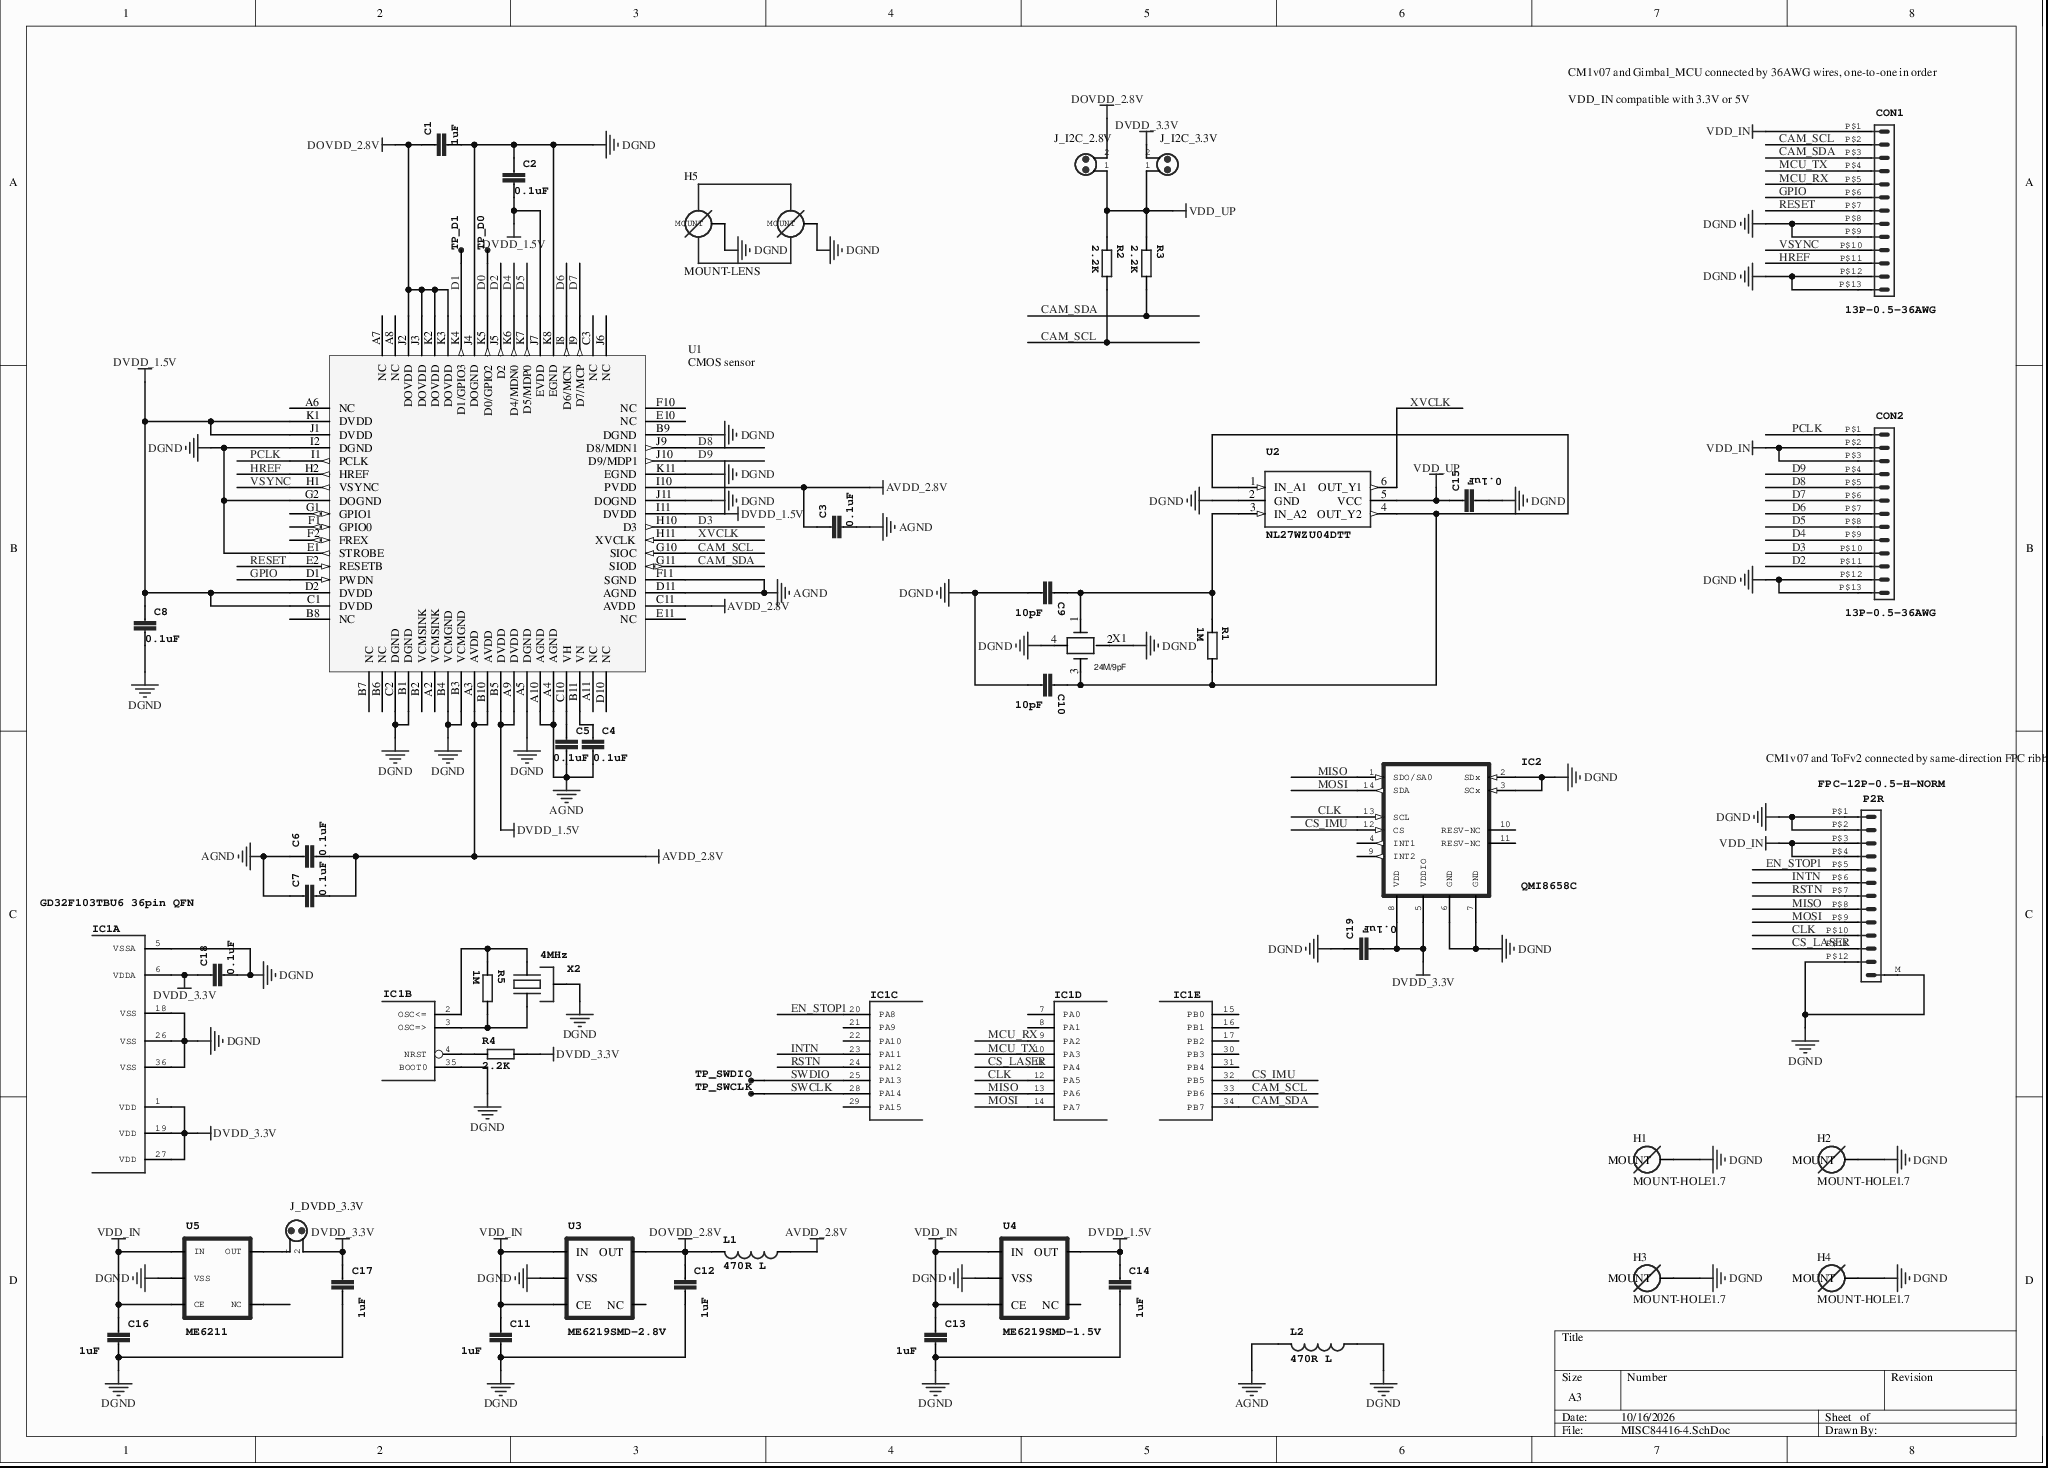
[diagram p0: MISC84416-4.SchDoc]
# Altium project MISC84416-3.PrjPcb
1 sheet, 50 parts. Net scope: global (net labels, ports and power ports of the same name join across sheets).
Board file: MISC84416.PcbDoc

## Sheet MISC84416-4.SchDoc
size A3

### Parts
C1  1uF  [RCL_C0402_TI]
C2  0.1uF  [RCL_C0402_TI]
C3  0.1uF  [RCL_C0402_TI]
C4  0.1uF  [RCL_C0402_TI]
C5  0.1uF  [RCL_C0402_TI]
C6  0.1uF  [RCL_C0402_TI]
C7  0.1uF  [RCL_C0402_TI]
C8  0.1uF  [RCL_C0402_TI]
C9  10pF  [RCL_C0402_TI]
C10  10pF  [RCL_C0402_TI]
C11  1uF  [RCL_C0402_TI]
C12  1uF  [RCL_C0402_TI]
C13  1uF  [RCL_C0402_TI]
C14  1uF  [RCL_C0402_TI]
C15  0.1uF  [RCL_C0402_TI]
C16  1uF  [RCL_C0402_TI]
C17  1uF  [RCL_C0402_TI]
C18  0.1uF  [RCL_C0402_TI]
C19  0.1uF  [RCL_C0402_TI]
CON1  13P-0.5-36AWG  [13P-0.5-36AWG]
CON2  13P-0.5-36AWG  [13P-0.5-36AWG]
H1  MOUNT-HOLE1.7  [MOUNT-HOLE1.7]
H2  MOUNT-HOLE1.7  [MOUNT-HOLE1.7]
H3  MOUNT-HOLE1.7  [MOUNT-HOLE1.7]
H4  MOUNT-HOLE1.7  [MOUNT-HOLE1.7]
H5  MOUNT-LENS  [MOUNT-LENS-M12-1.6]
IC1  GD32F103TBU6 36pin QFN  [GD32_QFN36]  (parts A,B,C,D,E of 5)
IC2  QMI8658C  [LGA14_3X2.5]
J_DVDD_3.3V  JUMPER_2P_MIN  [JUMPER_2P_MIN]  (value not drawn)
J_I2C_2.8V  JUMPER_2P_MIN  [JUMPER_2P_MIN]  (value not drawn)
J_I2C_3.3V  JUMPER_2P_MIN  [JUMPER_2P_MIN]  (value not drawn)
L1  470R L  [RCL_L0603]
L2  470R L  [RCL_L0603]
P2R  FPC-12P-0.5-H-NORM  [FPC-12P-0.5-H-NORM]
R1  1M  [RCL_R0402_TI]
R2  2.2K  [RCL_R0402_TI]
R3  2.2K  [RCL_R0402_TI]
R4  2.2K  [RCL_R0402_TI]
R5  1M  [RCL_R0402_TI]
TP_D0  (no value)  [TP-1]
TP_D1  (no value)  [TP-1]
TP_SWCLK  (no value)  [TP-1]
TP_SWDIO  (no value)  [TP-1]
U1  CMOS sensor  [BGA71_5.99X5.84]
U2  NL27WZU04DTT  [SOT23-6]
U3  ME6219SMD-2.8V  [SOT23-5]
U4  ME6219SMD-1.5V  [SOT23-5]
U5  ME6211  [SOT23-5]
X1  24M/9pF  [EPSON-TSX3225]
X2  4MHz  [XTAL_4.5X2.0]

### Nets
AGND: C3.2 C4.2 C5.2 C6.1 C7.1 L2.2 U1.A4(AGND) U1.A10(AGND) U1.D11(AGND) U1.F11(SGND)
AVDD_2.8V: C3.1 C6.2 C7.2 L1.1 U1.A3(AVDD) U1.B10(AVDD) U1.C11(AVDD) U1.I10(PVDD)
DGND: C1.2 C2.1 C8.2 C9.2 C10.2 C11.2 C12.2 C13.2 C14.2 C15.2 C16.2 C17.2 C18.2 C19.1 CON1.P$8 CON1.P$9 CON1.P$12 CON1.P$13 CON2.P$12 CON2.P$13 H1.MOUNT H2.MOUNT H3.MOUNT H4.MOUNT H5.MOUNT IC1.5(VSSA) IC1.18(VSS) IC1.26(VSS) IC1.35(BOOT0) IC1.36(VSS) IC2.2(SDx) IC2.3(SCx) IC2.6(GND) IC2.7(GND) L2.1 P2R.M P2R.P$1 P2R.P$2 P2R.P$12 U1.A5(DGND) U1.B1(DGND) U1.B3(VCMGND) U1.B4(VCMGND) U1.B9(DGND) U1.C2(DGND) U1.E1(STROBE) U1.G2(DOGND) U1.I2(DGND) U1.J4(DOGND) U1.J11(DOGND) U1.K8(EGND) U1.K11(EGND) U2.2(GND) U3.2(VSS) U4.2(VSS) U5.2(VSS) X1.2(Shield) X1.4(Shield) X2.2
DOVDD_2.8V: C1.1 C12.1 J_I2C_2.8V.2 L1.2 U1.J2(DOVDD) U1.J3(DOVDD) U1.K2(DOVDD) U1.K3(DOVDD) U3.5(OUT)
DVDD_1.5V: C2.2 C8.1 C14.1 U1.A9(DVDD) U1.B5(DVDD) U1.C1(DVDD) U1.D2(DVDD) U1.I11(DVDD) U1.J1(DVDD) U1.J7(EVDD) U1.K1(DVDD) U4.5(OUT)
DVDD_3.3V: C17.1 C18.1 C19.2 IC1.1(VDD) IC1.6(VDDA) IC1.19(VDD) IC1.27(VDD) IC2.5(VDDIO) IC2.8(VDD) J_DVDD_3.3V.2 J_I2C_3.3V.2 R4.2
VDD_IN: C11.1 C13.1 C16.1 CON1.P$1 CON2.P$2 CON2.P$3 P2R.P$3 P2R.P$4 U3.1(IN) U3.3(CE) U4.1(IN) U4.3(CE) U5.1(IN) U5.3(CE)
VDD_UP: C15.1 J_I2C_2.8V.1 J_I2C_3.3V.1 R2.1 R3.1 U2.5(VCC)
CAM_SCL: CON1.P$2 IC1.33(PB6) R2.2 U1.G10(SIOC)
CAM_SDA: CON1.P$3 IC1.34(PB7) R3.2 U1.G11(SIOD)
CLK: IC1.12(PA5) IC2.13(SCL) P2R.P$10
CS_IMU: IC1.32(PB5) IC2.12(CS)
CS_LASER: IC1.11(PA4) P2R.P$11
D0: TP_D0.1 U1.K5(D0/GPIO2)
D1: TP_D1.1 U1.K4(D1/GPIO3)
D2: CON2.P$11 U1.J5(D2)
D3: CON2.P$10 U1.H10(D3)
D4: CON2.P$9 U1.K6(D4/MDN0)
D5: CON2.P$8 U1.K7(D5/MDP0)
D6: CON2.P$7 U1.I8(D6/MCN)
D7: CON2.P$6 U1.I9(D7/MCP)
D8: CON2.P$5 U1.J9(D8/MDN1)
D9: CON2.P$4 U1.J10(D9/MDP1)
EN_STOP1: IC1.20(PA8) P2R.P$5
GPIO: CON1.P$6 U1.D1(PWDN)
HREF: CON1.P$11 U1.H2(HREF)
INTN: IC1.23(PA11) P2R.P$6
MCU_RX: CON1.P$5 IC1.9(PA2)
MCU_TX: CON1.P$4 IC1.10(PA3)
MISO: IC1.13(PA6) IC2.1(SDO/SA0) P2R.P$8
MOSI: IC1.14(PA7) IC2.14(SDA) P2R.P$9
PCLK: CON2.P$1 U1.I1(PCLK)
RESET: CON1.P$7 U1.E2(RESETB)
RSTN: IC1.24(PA12) P2R.P$7
SWCLK: IC1.28(PA14) TP_SWCLK.1
SWDIO: IC1.25(PA13) TP_SWDIO.1
VSYNC: CON1.P$10 U1.H1(VSYNC)
XVCLK: U1.H11(XVCLK) U2.6(OUT_Y1)
NetC4_1: C4.1 U1.B11(VN)
NetC5_1: C5.1 U1.C10(VH)
NetC9_1: C9.1 R1.1 U2.3(IN_A2) X1.1
NetC10_1: C10.1 R1.2 U2.1(IN_A1) U2.4(OUT_Y2) X1.3
NetIC1_2: IC1.2(OSC<=) R5.1 X2.3
NetIC1_3: IC1.3(OSC=>) R5.2 X2.1
NetIC1_4: IC1.4(NRST) R4.1
NetJ_DVDD_3.3V_1: J_DVDD_3.3V.1 U5.5(OUT)

Not connected (* = marked no-connect by the designer): IC1 7(PA0)* 8(PA1)* 15(PB0)* 16(PB1)* 17(PB2)* 21(PA9)* 22(PA10)* 29(PA15)* 30(PB3)* 31(PB4)*; IC2 4(INT1)* 9(INT2)* 10(RESV-NC)* 11(RESV-NC)*; U1 A2(VCMSINK)* A6(NC)* A7(NC)* A8(NC)* A11(NC)* B2(VCMSINK)* B6(NC)* B7(NC)* B8(NC)* C3(NC)* D10(NC)* E10(NC)* E11(NC)* F1(GPIO0)* F2(FREX)* F10(NC)* G1(GPIO1)* J6(NC)*; U3 4(NC)*; U4 4(NC)*; U5 4(NC)*

### Notes on the sheet
- VDD_IN compatible with 3.3V or 5V
- CM1v07 and Gimbal_MCU connected by 36AWG wires, one-to-one in order
- CM1v07 and ToFv2 connected by same-direction FPC ribbon cable

### Library data of the parts
C1-C19 = RCL_C-EUC0402_TI
IC1 = GD32F103TBU6
L1 L2 = RCL_L-USL0603
R1-R5 = RCL_R-EUR0402_TI
TP_D0 TP_D1 TP_SWCLK TP_SWDIO = TP-1
U1 = OV5640: 1/4INCH
U3 U4 = ME6219SMD
U5 = ME6211SMD
X1 = XTAL_EPSON_3225
X2 = XTAL_MURATA-4.5X2.0